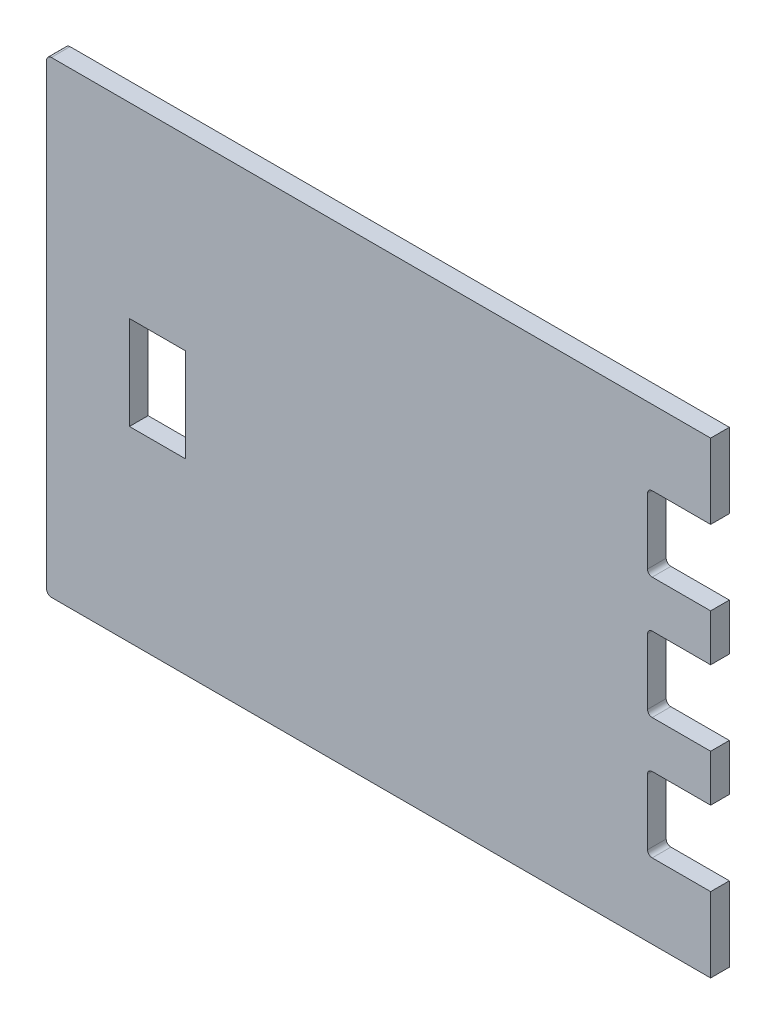
SolidWorks part; units mm, degrees
material "Q235B"
ref_plane "Front Plane" through (0, 0, 0) normal (0, 0, 1) x (1, 0, 0)
ref_plane "Top Plane" through (0, 0, 0) normal (0, 1, 0) x (1, 0, 0)
ref_plane "Right Plane" through (0, 0, 0) normal (1, 0, 0) x (0, 0, -1)
sketch "Sketch1" plane through (0, 0, 0) normal (0, 0, 1) x (1, 0, 0)
  line L0 (1420, 840) -> (1295, 840)
  line L1 (0, 0) -> (1420, 0)
  line L2 (0, 0) -> (0, 1000)
  line L3 (0, 1000) -> (1420, 1000)
  line L4 (1420, 0) -> (1420, 160)
  line L5 (1285, 830) -> (1285, 690)
  line L6 (1295, 680) -> (1420, 680)
  line L7 (1420, 840) -> (1420, 1000)
  line L8 (1295, 420) -> (1420, 420)
  line L9 (1420, 580) -> (1295, 580)
  line L10 (1285, 570) -> (1285, 430)
  line L11 (1295, 160) -> (1420, 160)
  line L12 (1420, 320) -> (1295, 320)
  line L13 (1285, 310) -> (1285, 170)
  line L14 (1420, 580) -> (1420, 680)
  line L15 (1420, 320) -> (1420, 420)
  line L17 (177, 600) -> (297, 600)
  line L18 (177, 600) -> (177, 400)
  line L19 (177, 400) -> (297, 400)
  line L20 (297, 600) -> (297, 400)
  arc A0 (1285, 690) -> (1295, 680) centre (1295, 690) ccw
  arc A1 (1295, 840) -> (1285, 830) centre (1295, 830) ccw
  arc A2 (1295, 580) -> (1285, 570) centre (1295, 570) ccw
  arc A3 (1285, 430) -> (1295, 420) centre (1295, 430) ccw
  arc A4 (1295, 320) -> (1285, 310) centre (1295, 310) ccw
  arc A5 (1285, 170) -> (1295, 160) centre (1295, 170) ccw
  point P13 (1285, 840)
  point P34 (237, 600)
  dimension "D6" = 10
  dimension "D1" = 1420
  dimension "D2" = 1000
  dimension "D3" = 160
  dimension "D4" = 135
  dimension "D5" = 160
  dimension "D8" = 120
  dimension "D9" = 1123
  dimension "D10" = 200
  dimension "D11" = 400
  dimension "D7" = 3
extrude "Boss-Extrude1" add sketch "Sketch1" along normal blind 40
fillet "Fillet1" radius 10 2 edges at (0, 0, 20) (0, 1000, 20)
